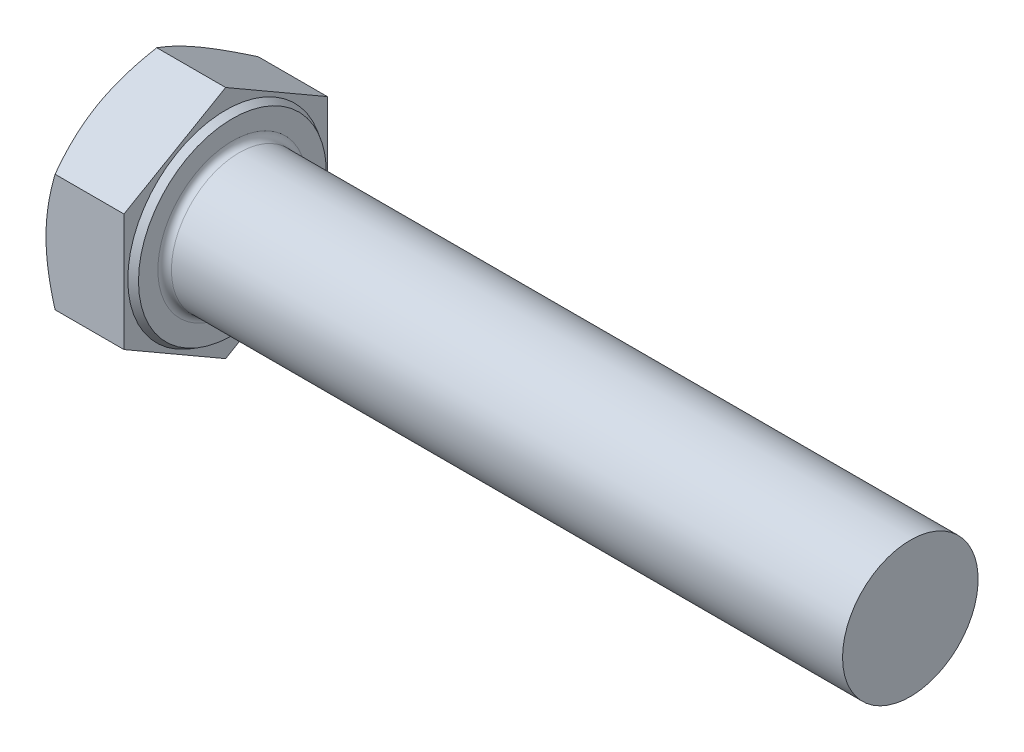
from build123d import *

# Parameters (mm, degrees)
EXTRUDE_387_DEPTH = 7.5
FILLET_1310_R     = 0.6


with BuildPart() as part:
    # 草图1 → Extrude 387 (new body)
    with BuildSketch(Plane(origin=(0, 0, 0), x_dir=(0, 0, -1), z_dir=(1, 0, 0))):
        Polygon((9, 5.196152423), (9, -5.196152423), (0, -10.392304845), (-9, -5.196152423), (-9, 5.196152423), (0, 10.392304845), align=None)
    extrude(amount=EXTRUDE_387_DEPTH)

    # 草图2 → 凸台-旋转1 (revolve)
    with BuildSketch(Plane.XY, mode=Mode.PRIVATE) as revolve_1_sk:
        Polygon((0, 0), (67.5, 0), (67.5, 4.4845), (67.5, 6), (37.5, 6), (0, 6), align=None)
    revolve(revolve_1_sk.sketch.rotate(Axis((0, 0, 0), (1, 0, 0)), 90), axis=Axis((0, 0, 0), (1, 0, 0)))

    # 草图3 → 切除-旋转1 (revolve, cut)
    with BuildSketch(Plane.XY):
        Polygon((0, 9), (3.690598923, 15.392304845), (3.690598923, 20.392304845), (-10, 20.392304845), (-10, 9), align=None)
    revolve(axis=Axis((0, 0, 0), (1, 0, 0)), mode=Mode.SUBTRACT)

    # 草图4 → 切除-旋转3 (revolve, cut)
    with BuildSketch(Plane.XY, mode=Mode.PRIVATE) as cut_revolve_3_sk:
        Polygon((7.5, 8.315), (6.9, 8.661410162), (6.9, 10.392304845), (7.5, 10.392304845), align=None)
    revolve(cut_revolve_3_sk.sketch.rotate(Axis((0, 0, 0), (1, 0, 0)), 90), axis=Axis((0, 0, 0), (1, 0, 0)), mode=Mode.SUBTRACT)

    # Fillet 1310
    fillet_1310_edges = [part.edges().sort_by_distance(p)[0] for p in [
        (7.5, 0, -6),
    ]]
    fillet(fillet_1310_edges, radius=FILLET_1310_R)


solid = part.part
